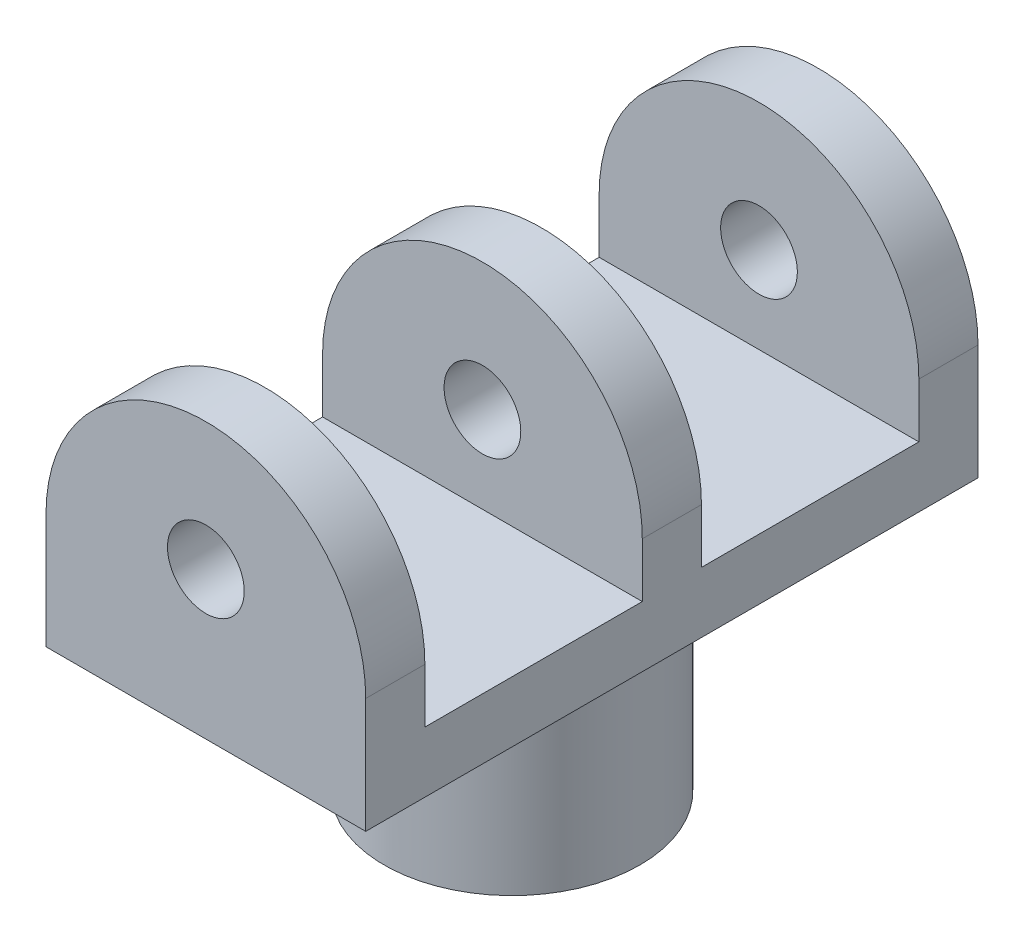
from build123d import *

# Parameters (mm, degrees)
SKETCH1_R               = 12
BOSS_EXTRUDE1_DEPTH     = 191.5
SKETCH2_R               = 40
BOSS_EXTRUDE2_DEPTH     = 62
SKETCH3_W               = 68
SKETCH3_H               = 67
CUT_EXTRUDE5_DEPTH      = 233.52580502
CUT_EXTRUDE8_DEPTH      = 233.52580502
CUT_EXTRUDE8_DEPTH_BACK = 233.52580502
SKETCH4_R               = 11


with BuildPart() as part:
    # Sketch1 → Boss-Extrude1 (new body)
    with BuildSketch(Plane.XY):
        with BuildLine():
            Line((0, 0), (0, 36))
            ThreePointArc((0, 36), (50, 86), (100, 36))
            Line((100, 36), (100, 0))
            Line((100, 0), (0, 0))
        make_face()
        with Locations((50, 46)):
            Circle(SKETCH1_R, mode=Mode.SUBTRACT)
    extrude(amount=BOSS_EXTRUDE1_DEPTH)

    # Sketch2 → Boss-Extrude2 (add)
    with BuildSketch(Plane(origin=(0, 0, 0), x_dir=(-1, 0, 0), z_dir=(0, -1, 0))):
        with Locations(Location((-50, -95.75, 0), (0, 0, 180))):
            Circle(SKETCH2_R)
    extrude(amount=BOSS_EXTRUDE2_DEPTH)

    # Sketch3 → Cut-Extrude5 (cut, through all)
    with BuildSketch(Plane(origin=(0, 0, 0), x_dir=(0, 0, -1), z_dir=(1, 0, 0))):
        with Locations((-52.5, 52.5)):
            Rectangle(SKETCH3_W, SKETCH3_H)
        with Locations((-139, 52.5)):
            Rectangle(SKETCH3_W, SKETCH3_H)
    extrude(amount=CUT_EXTRUDE5_DEPTH, mode=Mode.SUBTRACT)

    # Sketch4 → Cut-Extrude8 (cut, two sides: drawn at the far end of the back side and taken through both)
    with BuildSketch(Plane.XY.offset(-CUT_EXTRUDE8_DEPTH_BACK)):
        with Locations((50, -32)):
            Circle(SKETCH4_R)
    extrude(amount=CUT_EXTRUDE8_DEPTH + CUT_EXTRUDE8_DEPTH_BACK, mode=Mode.SUBTRACT)


solid = part.part
